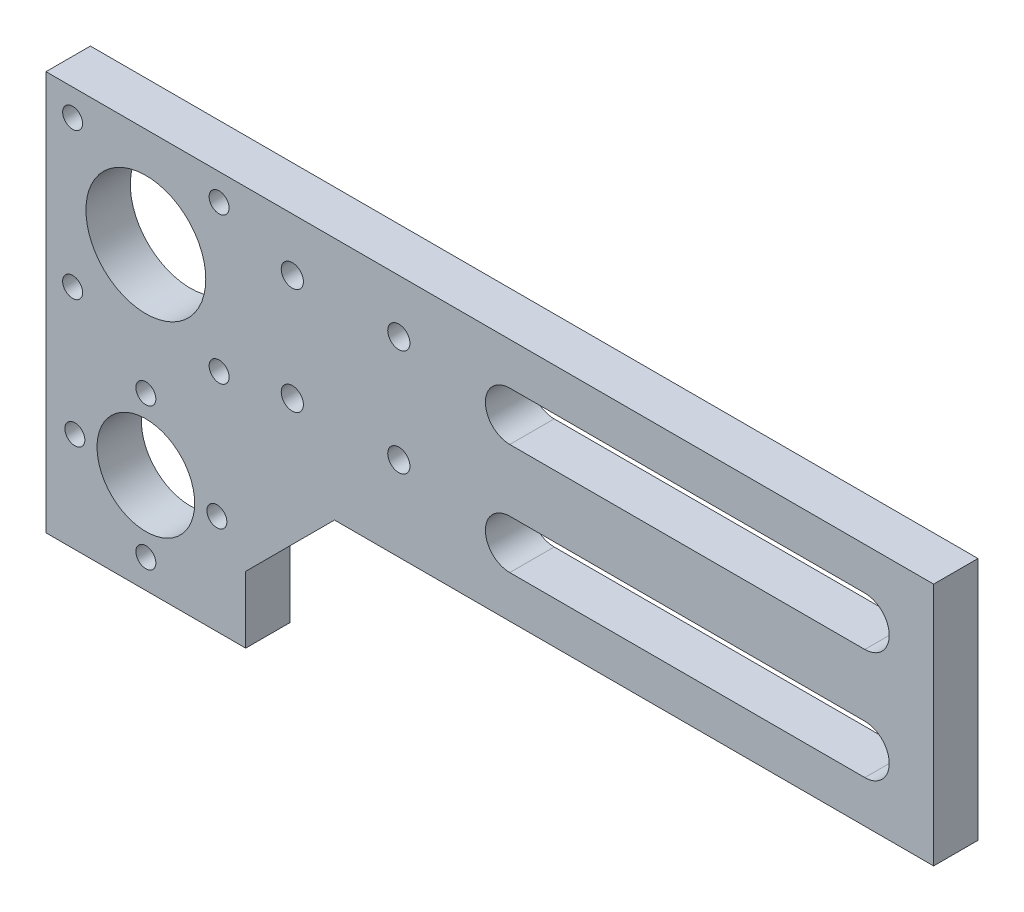
SolidWorks part; units mm, degrees
material "6061-O (GB)"
ref_plane "前视基准面" through (0, 0, 0) normal (0, 0, 1) x (1, 0, 0)
ref_plane "上视基准面" through (0, 0, 0) normal (0, 1, 0) x (1, 0, 0)
ref_plane "右视基准面" through (0, 0, 0) normal (1, 0, 0) x (0, 0, -1)
sketch "草图1" plane through (0, 0, 0) normal (0, 0, 1) x (1, 0, 0)
  line L0 (-22.5, 45) -> (0, 45) construction
  line L1 (-22.5, 67.5) -> (22.5, 67.5)
  line L2 (-22.5, 67.5) -> (-22.5, 22.5)
  line L3 (-22.5, 22.5) -> (22.5, 22.5)
  line L4 (22.5, 67.5) -> (22.5, 22.5)
  line L5 (0, 45) -> (0, 67.5) construction
  circle A0 centre (0, 0) radius 21
  circle A1 centre (0, 16) radius 2.25
  circle A2 centre (0, 0) radius 10.5
  point P11 (0, 22.5)
  dimension "D1" = 21
  dimension "D2" = 42
  dimension "D3" = 4.5
  dimension "D4" = 16
  dimension "D5" = 45
  dimension "D6" = 45
sketch "草图2" plane through (0, 0, 0) normal (0, 0, 1) x (1, 0, 0)
  line L0 (-22.5, 67.5) -> (177.5, 67.5)
  line L1 (177.5, 67.5) -> (177.5, 12.5)
  line L2 (177.5, 12.5) -> (22.5, 12.5)
  line L3 (22.5, 12.5) -> (22.5, -22.5)
  line L4 (22.5, -22.5) -> (-22.5, -22.5)
  line L5 (-22.5, -22.5) -> (-22.5, 67.5)
  line L6 (162, 52.5) -> (82, 52.5) construction
  line L7 (162, 47) -> (82, 47)
  line L8 (162, 58) -> (82, 58)
  line L9 (22.5, 45) -> (0, 45) construction
  line L10 (22.5, 67.5) -> (22.5, 22.5) construction
  line L11 (0, 45) -> (0, 67.5) construction
  line L12 (177.5, 40) -> (83.9226, 40) construction
  line L13 (162, 27.5) -> (82, 27.5) construction
  line L14 (162, 33) -> (82, 33)
  line L15 (162, 22) -> (82, 22)
  arc A0 (162, 47) -> (162, 58) centre (162, 52.5) ccw
  arc A1 (82, 58) -> (82, 47) centre (82, 52.5) ccw
  circle A3 centre (0, 0) radius 11
  circle A4 centre (0, 45) radius 13.5
  circle A5 centre (-16.5, 61.5) radius 2.25
  circle A6 centre (16.5, 61.5) radius 2.25
  circle A7 centre (16.5, 28.5) radius 2.25
  circle A8 centre (-16.5, 28.5) radius 2.25
  circle A9 centre (0, 16) radius 2.25 construction
  circle A10 centre (0, 16) radius 2.25
  circle A11 centre (16, 0) radius 2.25
  circle A12 centre (0, -16) radius 2.25
  circle A13 centre (-16, 0) radius 2.25
  arc A14 (162, 33) -> (162, 22) centre (162, 27.5) cw
  arc A15 (82, 22) -> (82, 33) centre (82, 27.5) cw
  point P10 (122, 52.5)
  point P15 (167.5, 52.5)
  point P46 (0, 0)
  point P47 (122, 27.5)
  dimension "D6" = 22
  dimension "D7" = 27
  dimension "D8" = 33
  dimension "D9" = 33
  dimension "D10" = 4.5
  dimension "D1" = 90
  dimension "D2" = 200
  dimension "D3" = 80
  dimension "D4" = 11
  dimension "D5" = 10
  dimension "D12" = 25
  dimension "D13" = 55
  dimension "D11" = 4
extrude "凸台-拉伸1" add sketch "草图2" along normal blind 10
chamfer "倒角1" distance 20 angle 45 1 edges at (22.5, 12.5, 5)
sketch "草图3" plane through (0, 0, 0) normal (0, 0, -1) x (-1, 0, 0)
  line L6 (-177.5, 67.5) -> (22.5, 67.5) construction
  line L7 (-68.5, 43.5) -> (-21.5, 43.5) construction
  line L8 (-45, 43.5) -> (-45, 67.5) construction
  circle A0 centre (-57, 55.5) radius 2.5
  circle A1 centre (-33, 55.5) radius 2.5
  circle A2 centre (-33, 31.5) radius 2.5
  circle A3 centre (-57, 31.5) radius 2.5
  dimension "D4" = 24
  dimension "D5" = 24
  dimension "D6" = 5
  dimension "D2" = 13.5
  dimension "D1" = 33
extrude "切除-拉伸1" cut sketch "草图3" against normal up to next
